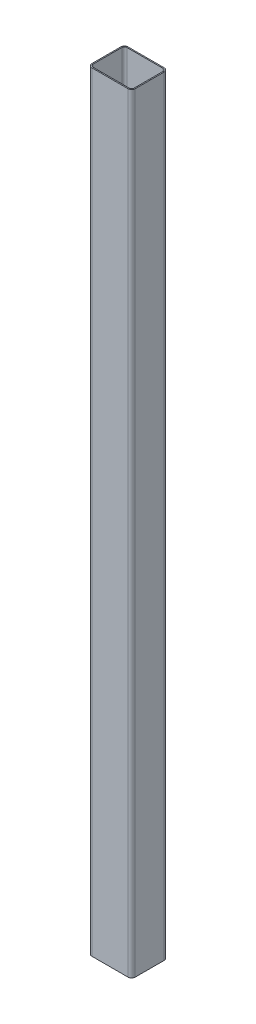
from build123d import *

# Parameters (mm, degrees)
EXTRUDE_THIN1_DEPTH = 1062


with BuildPart() as part:
    # Sketch1 → Extrude-Thin1 (new, symmetric)
    with BuildSketch(Plane(origin=(0, 0, 0), x_dir=(1, 0, 0), z_dir=(0, 1, 0))):
        with BuildLine():
            Line((-50, 50), (50, 50))
            ThreePointArc((50, 50), (57.071067812, 47.071067812), (60, 40))
            Line((60, 40), (60, -40))
            ThreePointArc((60, -40), (57.071067812, -47.071067812), (50, -50))
            Line((50, -50), (-50, -50))
            ThreePointArc((-50, -50), (-57.071067812, -47.071067812), (-60, -40))
            Line((-60, -40), (-60, 40))
            ThreePointArc((-60, 40), (-57.071067812, 47.071067812), (-50, 50))
        make_face()
        with BuildLine():
            Line((-50, 47), (50, 47))
            ThreePointArc((50, 47), (54.949747468, 44.949747468), (57, 40))
            Line((57, 40), (57, -40))
            ThreePointArc((57, -40), (54.949747468, -44.949747468), (50, -47))
            Line((50, -47), (-50, -47))
            ThreePointArc((-50, -47), (-54.949747468, -44.949747468), (-57, -40))
            Line((-57, -40), (-57, 40))
            ThreePointArc((-57, 40), (-54.949747468, 44.949747468), (-50, 47))
        make_face(mode=Mode.SUBTRACT)
    extrude(amount=EXTRUDE_THIN1_DEPTH, both=True)


solid = part.part
